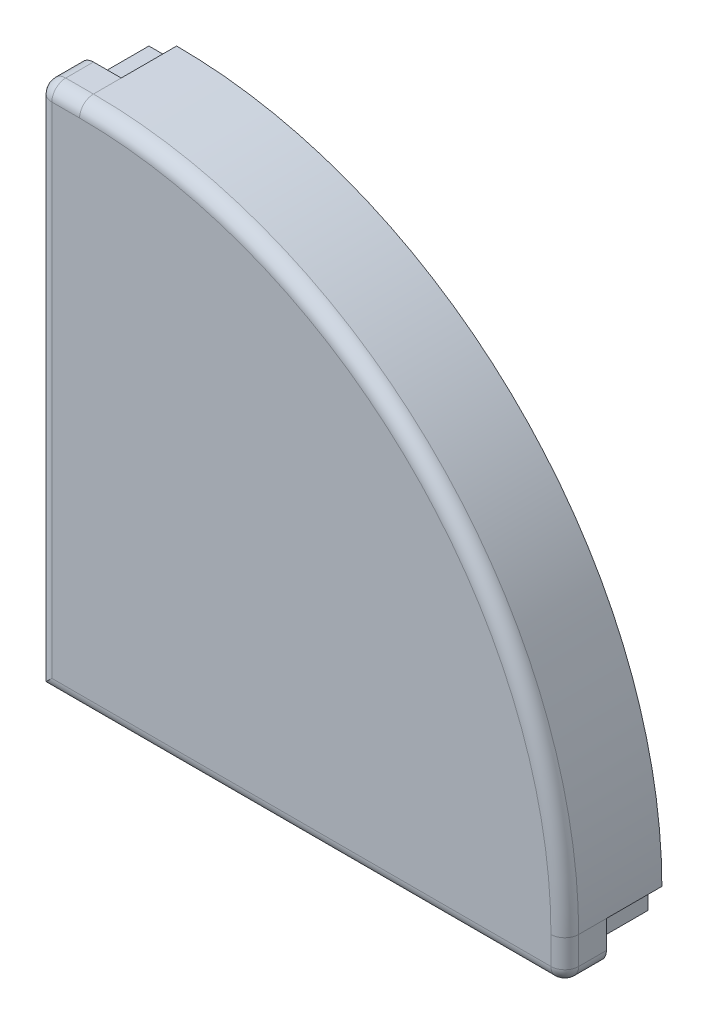
SolidWorks part; units mm, degrees
ref_plane "Frontal" through (0, 0, 0) normal (0, 0, 1) x (1, 0, 0)
ref_plane "Superior" through (0, 0, 0) normal (0, 1, 0) x (1, 0, 0)
ref_plane "Direito" through (0, 0, 0) normal (1, 0, 0) x (0, 0, -1)
sketch "Sketch1" plane through (0, 0, 0) normal (0, 0, 1) x (1, 0, 0)
  line L0 (0, 0) -> (0, 19)
  line L1 (19, 0) -> (0, 0)
  line L2 (0, 19) -> (1.5, 19)
  line L3 (19, 1.5) -> (19, 0)
  arc A0 (1.5, 19) -> (19, 1.5) centre (1.5, 1.5) cw
  dimension "D1" = 19
  dimension "D2" = 1.5
  dimension "D3" = 1.5
extrude "Boss-Extrude1" add sketch "Sketch1" along normal blind 1.5
sketch "Sketch2" plane through (0, 0, 0) normal (0, 0, 1) x (1, 0, 0)
  line L0 (1.5, 19) -> (1.5, 18.5)
  line L1 (1.5, 18.5) -> (0.5, 18.5)
  line L2 (0.5, 18.5) -> (0.5, 17.5)
  line L3 (0.5, 17.5) -> (1.5, 17.5)
  line L4 (17.5, 1.5) -> (17.5, 0.5)
  line L5 (17.5, 0.5) -> (18.5, 0.5)
  line L6 (18.5, 0.5) -> (18.5, 1.5)
  line L7 (18.5, 1.5) -> (19, 1.5)
  line L8 (1.5, 16.5) -> (1.5, 0)
  line L9 (0, 0) -> (19, 0) construction
  line L10 (1.5, 0) -> (1.5, 16.5) construction
  line L11 (1.5, 0) -> (16.5, 0)
  line L12 (16.5, 1.5) -> (16.5, 0) construction
  line L13 (16.5, 0) -> (16.5, 1.5)
  line L14 (3, 14.9164) -> (3, 1.5)
  line L15 (3, 1.5) -> (15, 1.5)
  line L16 (15, 1.5) -> (15, 1.5)
  arc A0 (1.5, 17.5) -> (17.5, 1.5) centre (1.5, 1.5) cw
  arc A1 (19, 1.5) -> (1.5, 19) centre (1.5, 1.5) ccw
  arc A2 (16.5, 1.5) -> (1.5, 16.5) centre (1.5, 1.5) ccw
  arc A3 (15, 1.5) -> (3, 14.9164) centre (1.5, 1.5) ccw
  dimension "D1" = 1.5
extrude "Boss-Extrude3" add sketch "Sketch2" against normal blind 2
fillet "Filete1" radius 0.5 7 edges at (19, 0.75, 1.5) (0.75, 19, 1.5) (0, 19, 0.75) (19, 0, 0.75) (9.5, 0, 1.5) (0, 9.5, 1.5) (13.8744, 13.8744, 1.5)
